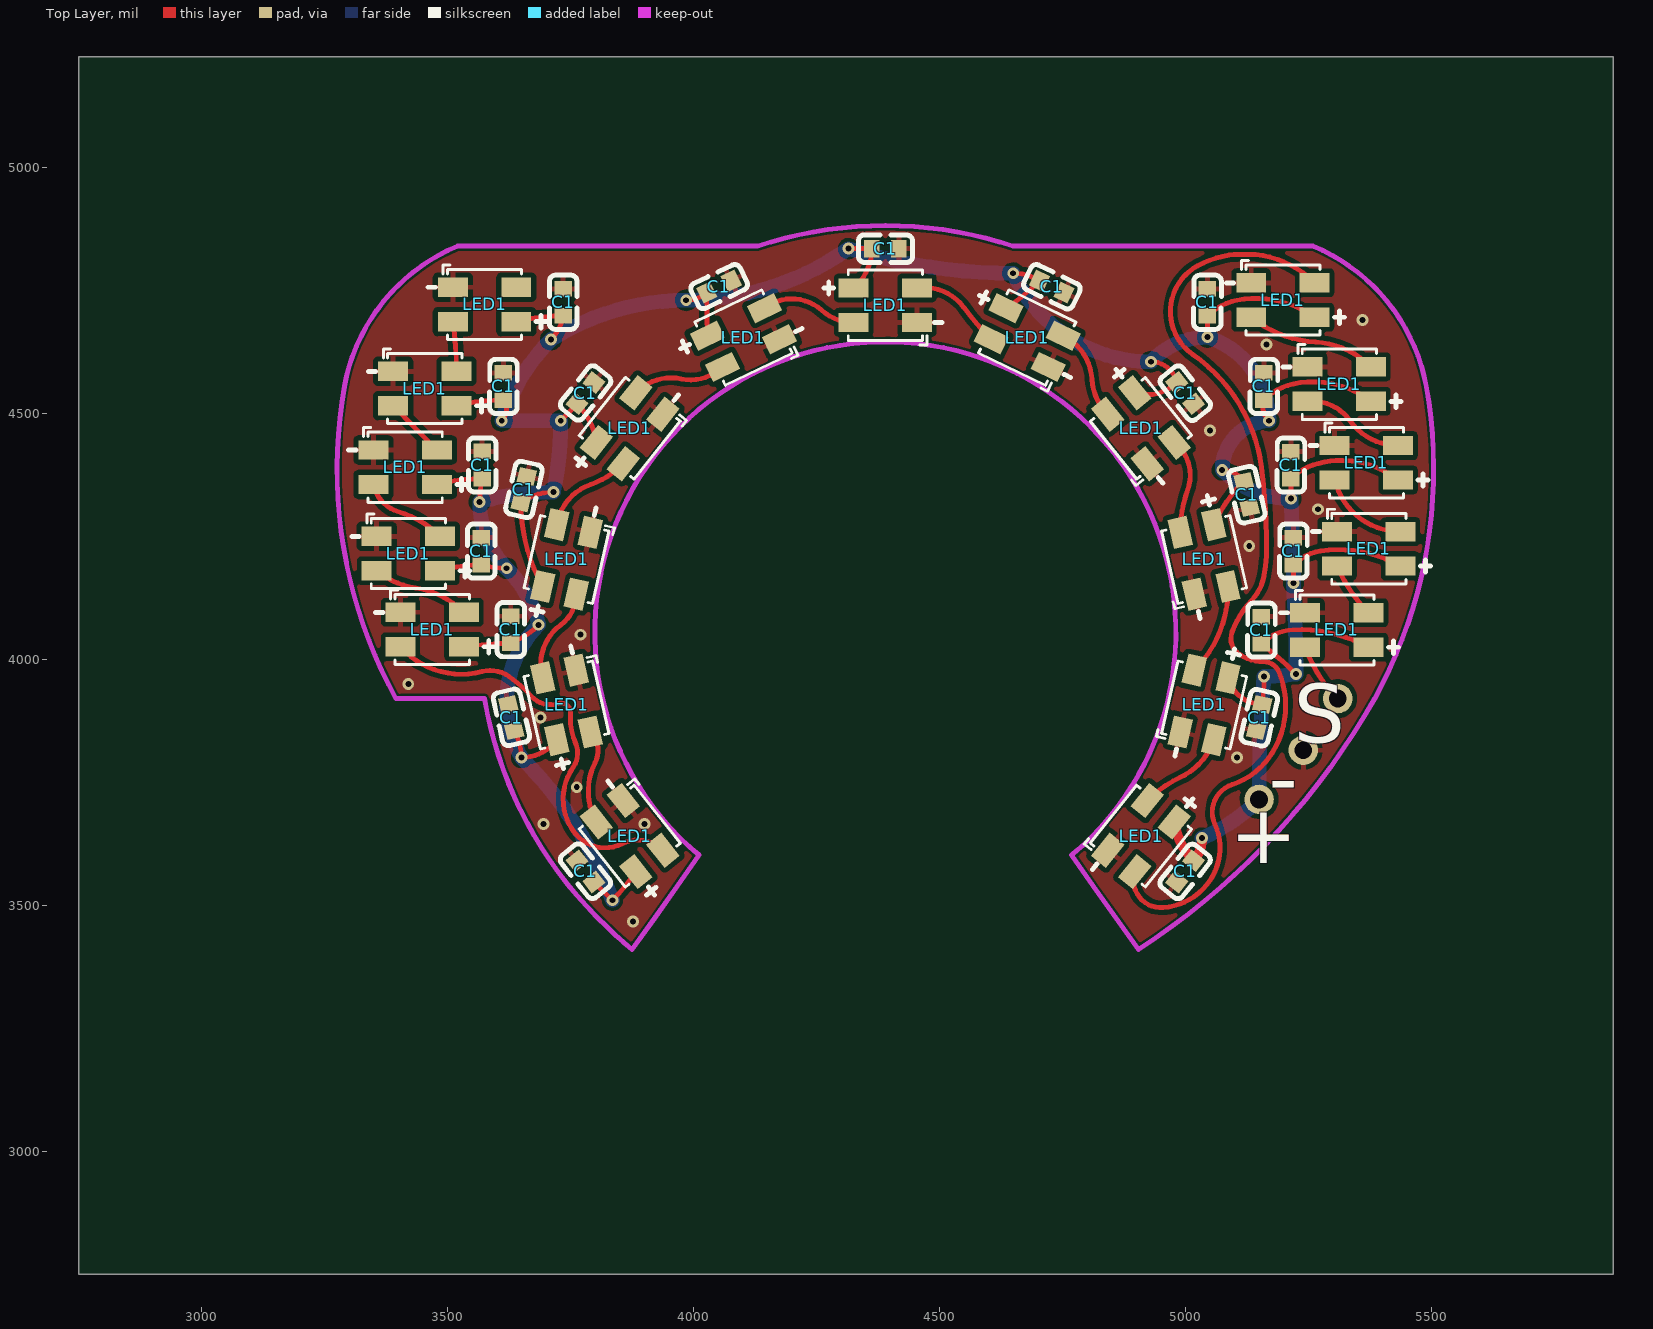
[diagram p0: Top Layer view]
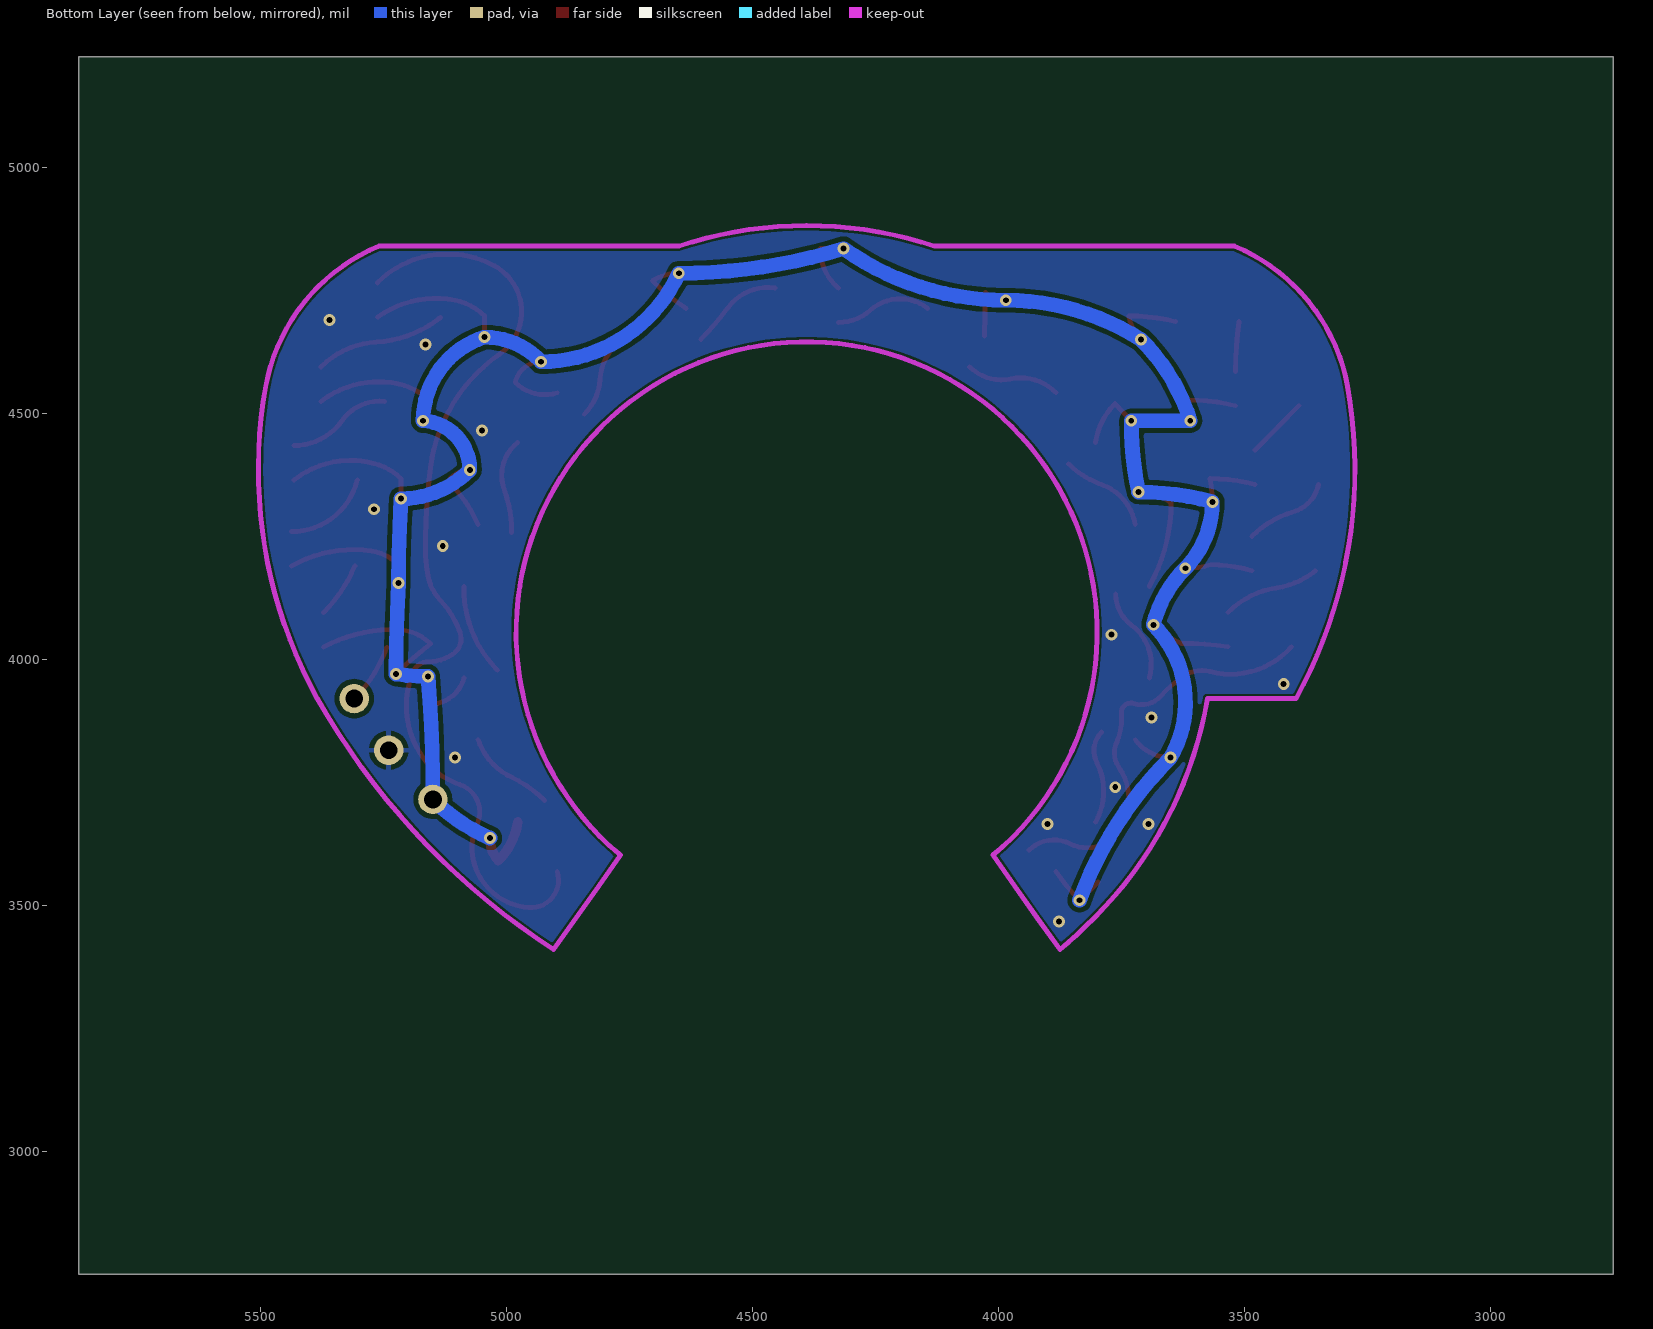
[diagram p1: Bottom Layer view, seen from below]
# Altium PCB MISC89036.pcbdoc
Units mil, origin at the board's own origin, x right, y up, seen from the top; angles counter-clockwise.
Board outline 3120 x 2475.23 mil, 2 copper layers (Top Layer, Bottom Layer), stack 62.206 mil thick; 42 components, 2 nets, 129 pads, 34 vias.

## Layer stack, top to bottom
Top Solder Mask Layer: solder mask 0.394, Dk 3.3
Top Layer: signal copper 1.379
Dielectric1: surface 59.449, FR4, Dk 4.5
Bottom Layer: signal copper 1.378
Bottom Solder Mask Layer: solder mask 0.394, Dk 3.3

## Board outline
5870,2750 2750,2750 2750,5225.23 5870,5225.23

## Design rules (kind name [scope] priority, off if disabled: settings)
BoardOutlineClearance copperThickness2oz_1 [All] p2 off: genericclearance=7.99 ignorepadtopadclearanceinfootprint=FALSE except(0: Arc-SplitContinuation Track-SplitContinuation SMDPad-SplitContinuation THPad-SplitContinuation Via-SplitContinuation Fill-SplitContinuation Region-SplitContinuation Poly-SplitContinuation Text-SplitContinuation Hole-SplitContinuation; 5.98: Arc-CutoutEdge Track-CutoutEdge SMDPad-CutoutEdge THPad-CutoutEdge Via-CutoutEdge Text-CutoutEdge; 6.9: Hole-OutlineEdge Hole-CutoutEdge; 10: Poly-OutlineEdge Poly-CutoutEdge; 11.81: Arc-OutlineEdge Track-OutlineEdge SMDPad-OutlineEdge THPad-OutlineEdge Via-OutlineEdge Fill-OutlineEdge Region-OutlineEdge Text-OutlineEdge Fill-CutoutEdge Region-CutoutEdge)
BoardOutlineClearance Plane_innerPlane_1 [All] p4 off: genericclearance=4.02 ignorepadtopadclearanceinfootprint=FALSE except(0: Arc-SplitContinuation Track-SplitContinuation SMDPad-SplitContinuation THPad-SplitContinuation Via-SplitContinuation Fill-SplitContinuation Region-SplitContinuation Poly-SplitContinuation Text-SplitContinuation Hole-SplitContinuation; 5.98: Arc-CutoutEdge Track-CutoutEdge SMDPad-CutoutEdge THPad-CutoutEdge Via-CutoutEdge Text-CutoutEdge; 6.9: Hole-OutlineEdge Hole-CutoutEdge; 10: Poly-OutlineEdge Poly-CutoutEdge; 11.81: Arc-OutlineEdge Track-OutlineEdge SMDPad-OutlineEdge THPad-OutlineEdge Via-OutlineEdge Fill-OutlineEdge Region-OutlineEdge Text-OutlineEdge Fill-CutoutEdge Region-CutoutEdge)
BoardOutlineClearance Copper_copperRegion_1 [All] p6 off: genericclearance=4.02 ignorepadtopadclearanceinfootprint=FALSE except(0: Arc-SplitContinuation Track-SplitContinuation SMDPad-SplitContinuation THPad-SplitContinuation Via-SplitContinuation Fill-SplitContinuation Region-SplitContinuation Poly-SplitContinuation Text-SplitContinuation Hole-SplitContinuation; 5.98: Arc-CutoutEdge Track-CutoutEdge SMDPad-CutoutEdge THPad-CutoutEdge Via-CutoutEdge Text-CutoutEdge; 6.9: Hole-OutlineEdge Hole-CutoutEdge; 10: Poly-OutlineEdge Poly-CutoutEdge; 11.81: Arc-OutlineEdge Track-OutlineEdge SMDPad-OutlineEdge THPad-OutlineEdge Via-OutlineEdge Fill-OutlineEdge Region-OutlineEdge Text-OutlineEdge Fill-CutoutEdge Region-CutoutEdge)
BoardOutlineClearance copperThickness1oz_1 [All] p8: genericclearance=4.02 ignorepadtopadclearanceinfootprint=FALSE except(0: Arc-SplitContinuation Track-SplitContinuation SMDPad-SplitContinuation THPad-SplitContinuation Via-SplitContinuation Fill-SplitContinuation Region-SplitContinuation Poly-SplitContinuation Text-SplitContinuation Hole-SplitContinuation; 5.98: Arc-CutoutEdge Track-CutoutEdge SMDPad-CutoutEdge THPad-CutoutEdge Via-CutoutEdge Text-CutoutEdge; 6.9: Hole-OutlineEdge Hole-CutoutEdge; 10: Poly-OutlineEdge Poly-CutoutEdge; 11.81: Arc-OutlineEdge Track-OutlineEdge SMDPad-OutlineEdge THPad-OutlineEdge Via-OutlineEdge Fill-OutlineEdge Region-OutlineEdge Text-OutlineEdge Fill-CutoutEdge Region-CutoutEdge)
Clearance copperThickness2oz [All] p1 off: gap=7.99 ignorepadtopadclearanceinfootprint=FALSE except(5.98: SMDPad-Track SMDPad-SMDPad THPad-Track SMDPad-THPad THPad-THPad Track-Via SMDPad-Via THPad-Via Via-Via Fill-SMDPad Region-SMDPad Fill-THPad Region-THPad Fill-Via Region-Via Fill-Fill Fill-Region Region-Region Arc-Track Arc-SMDPad Arc-THPad Arc-Via Fill-Arc Region-Arc Arc-Arc Text-Track SMDPad-Text Text-THPad Text-Via Fill-Text Region-Text Arc-Text Text-Text; 6.9: Hole-Track Hole-SMDPad Hole-THPad Hole-Via Fill-Hole Region-Hole Hole-Arc Hole-Text; 10: Poly-Track Poly-SMDPad Poly-THPad Poly-Via Poly-Fill Poly-Region Poly-Poly Poly-Arc Poly-Text Poly-Hole; 11.81: Fill-Track Region-Track)
Clearance Plane_innerPlane [All] p3 off: gap=4.02 ignorepadtopadclearanceinfootprint=FALSE except(5.98: SMDPad-Track SMDPad-SMDPad THPad-Track SMDPad-THPad THPad-THPad Track-Via SMDPad-Via THPad-Via Via-Via Fill-SMDPad Region-SMDPad Fill-THPad Region-THPad Fill-Via Region-Via Fill-Fill Fill-Region Region-Region Arc-Track Arc-SMDPad Arc-THPad Arc-Via Fill-Arc Region-Arc Arc-Arc Text-Track SMDPad-Text Text-THPad Text-Via Fill-Text Region-Text Arc-Text Text-Text; 6.9: Hole-Track Hole-SMDPad Hole-THPad Hole-Via Fill-Hole Region-Hole Hole-Arc Hole-Text; 10: Poly-Track Poly-SMDPad Poly-THPad Poly-Via Poly-Fill Poly-Region Poly-Poly Poly-Arc Poly-Text Poly-Hole; 11.81: Fill-Track Region-Track)
Clearance Copper_copperRegion [All] p5 off: gap=4.02 ignorepadtopadclearanceinfootprint=FALSE except(5.98: SMDPad-Track SMDPad-SMDPad THPad-Track SMDPad-THPad THPad-THPad Track-Via SMDPad-Via THPad-Via Via-Via Fill-SMDPad Region-SMDPad Fill-THPad Region-THPad Fill-Via Region-Via Fill-Fill Fill-Region Region-Region Arc-Track Arc-SMDPad Arc-THPad Arc-Via Fill-Arc Region-Arc Arc-Arc Text-Track SMDPad-Text Text-THPad Text-Via Fill-Text Region-Text Arc-Text Text-Text; 6.9: Hole-Track Hole-SMDPad Hole-THPad Hole-Via Fill-Hole Region-Hole Hole-Arc Hole-Text; 10: Poly-Track Poly-SMDPad Poly-THPad Poly-Via Poly-Fill Poly-Region Poly-Poly Poly-Arc Poly-Text Poly-Hole; 11.81: Fill-Track Region-Track)
Clearance copperThickness1oz [All] p7: gap=4.02 ignorepadtopadclearanceinfootprint=FALSE except(5.98: SMDPad-Track SMDPad-SMDPad THPad-Track SMDPad-THPad THPad-THPad Track-Via SMDPad-Via THPad-Via Via-Via Fill-SMDPad Region-SMDPad Fill-THPad Region-THPad Fill-Via Region-Via Fill-Fill Fill-Region Region-Region Arc-Track Arc-SMDPad Arc-THPad Arc-Via Fill-Arc Region-Arc Arc-Arc Text-Track SMDPad-Text Text-THPad Text-Via Fill-Text Region-Text Arc-Text Text-Text; 6.9: Hole-Track Hole-SMDPad Hole-THPad Hole-Via Fill-Hole Region-Hole Hole-Arc Hole-Text; 10: Poly-Track Poly-SMDPad Poly-THPad Poly-Via Poly-Fill Poly-Region Poly-Poly Poly-Arc Poly-Text Poly-Hole; 11.81: Fill-Track Region-Track)
DiffPairsRouting differentialPair [All] p1: maxlimit=6 minlimit=6 mostfreqgap=6 toplayer_minwidth=5 toplayer_prefwidth=10 toplayer_maxwidth=100 toplayer_mingap=6 toplayer_prefgap=6 toplayer_maxgap=6 bottomlayer_minwidth=5 bottomlayer_prefwidth=10 bottomlayer_maxwidth=100 bottomlayer_mingap=6 bottomlayer_prefgap=6 bottomlayer_maxgap=6 maxuncoupledlength=10
HoleToHoleClearance otherClearance [All] p1: gap=11.81 allowstackedmicrovias=TRUE
Length netLength [All] p1: minlimit=0 maxlimit=0
PasteMaskExpansion pasteMaskExpansion [All] p1: expansion=0
PlaneConnect innerPlane [All] p1: planeconnectstyle=Relief reliefexpansion=20 reliefentries=4 reliefconductorwidth=10 reliefairgap=10
PolygonConnect copperRegion [All] p1: connectstyle=Relief reliefconductorwidth=10 reliefentries=4 polygonreliefangle="90 Angle" airgapwidth=10 via.connectstyle=Relief via.reliefconductorwidth=10 via.reliefentries=4 via.polygonreliefangle="90 Angle" via.airgapwidth=10
RoutingVias viaSize [All] p1: holewidth=12.01 width=24.02 viastyle="Through Hole" minholewidth=11.81 minwidth=19.68 maxholewidth=248.03 maxwidth=393.7
SolderMaskExpansion solderMaskExpansion [IsVia] p1: expansion=-1000 istentingtop=TRUE
SolderMaskExpansion solderMaskExpansion [All] p2: expansion=2 istentingtop=FALSE
Width copperThickness2oz_2 [All] p1 off: maxlimit=100 minlimit=8 preferedwidth=10
Width copperThickness1oz_2 [All] p2: maxlimit=100 minlimit=5 preferedwidth=10

## Components (designator, comment, footprint, x,y, rotation, side; value= is the part's Value field where it differs from the comment)
C1 "100nF" C0603#1 4390,4835.23 r180 top
C1 "100nF" C0603#2 4051.57,4757.99 r205.7 top
C1 "100nF" C0603#3 3780.17,4541.55 r231.4 top
C1 "100nF" C0603#4 3655,4345.23 r257.1 top
C1 "100nF" C0603#5 3629.56,3881.66 r282.9 top
C1 "100nF" C0603#6 3780.17,3568.91 r308.6 top
C1 "100nF" C0603#3 4999.83,3568.91 r51.4 top
C1 "100nF" C0603#4 5150.44,3881.66 r77.1 top
C1 "100nF" C0603#5 5125,4335.23 r102.9 top
C1 "100nF" C0603#6 4999.83,4541.55 r128.6 top
C1 "100nF" C0603#7 4728.43,4757.99 r154.3 top
C1 "100nF" C0603#1 3734.79,4725.92 r270 top
C1 "100nF" C0603#1 3613.31,4554.92 r270 top
C1 "100nF" C0603#1 3570,4395.23 r270 top
C1 "100nF" C0603#1 3568.31,4219.92 r270 top
C1 "100nF" C0603#1 3628.31,4060.12 r270 top
C1 "100nF" C0603#1 5045,4725.92 r270 top
C1 "100nF" C0603#1 5159.72,4554.92 r270 top
C1 "100nF" C0603#1 5214.72,4394.92 r270 top
C1 "100nF" C0603#1 5219.72,4219.92 r270 top
C1 "100nF" C0603#1 5154.72,4059.23 r270 top
LED1 "WS2812B-Mini" LED-SMD_4P-L3.5-W3.5-TL_WS2812B#1 4390,4720.23 r0 top
LED1 "WS2812B-Mini" LED-SMD_4P-L3.5-W3.5-TL_WS2812B#2 4101.47,4654.37 r25.7 top
LED1 "WS2812B-Mini" LED-SMD_4P-L3.5-W3.5-TL_WS2812B#3 3870.08,4469.85 r51.4 top
LED1 "WS2812B-Mini" LED-SMD_4P-L3.5-W3.5-TL_WS2812B#4 3741.67,4203.21 r77.1 top
LED1 "WS2812B-Mini" LED-SMD_4P-L3.5-W3.5-TL_WS2812B#5 3741.67,3907.25 r102.9 top
LED1 "WS2812B-Mini" LED-SMD_4P-L3.5-W3.5-TL_WS2812B#6 3870.08,3640.61 r128.6 top
LED1 "WS2812B-Mini" LED-SMD_4P-L3.5-W3.5-TL_WS2812B#3 4909.92,3640.61 r231.4 top
LED1 "WS2812B-Mini" LED-SMD_4P-L3.5-W3.5-TL_WS2812B#4 5038.33,3907.25 r257.1 top
LED1 "WS2812B-Mini" LED-SMD_4P-L3.5-W3.5-TL_WS2812B#5 5038.33,4203.21 r282.9 top
LED1 "WS2812B-Mini" LED-SMD_4P-L3.5-W3.5-TL_WS2812B#6 4909.92,4469.85 r308.6 top
LED1 "WS2812B-Mini" LED-SMD_4P-L3.5-W3.5-TL_WS2812B#7 4678.53,4654.37 r334.3 top
LED1 "WS2812B-Mini" LED-SMD_4P-L3.5-W3.5-TL_WS2812B#1 3575,4721.73 r180 top
LED1 "WS2812B-Mini" LED-SMD_4P-L3.5-W3.5-TL_WS2812B#1 3453.52,4550.73 r180 top
LED1 "WS2812B-Mini" LED-SMD_4P-L3.5-W3.5-TL_WS2812B#1 3413.52,4390.73 r180 top
LED1 "WS2812B-Mini" LED-SMD_4P-L3.5-W3.5-TL_WS2812B#1 3420,4215.23 r180 top
LED1 "WS2812B-Mini" LED-SMD_4P-L3.5-W3.5-TL_WS2812B#1 3468.52,4060.73 r180 top
LED1 "WS2812B-Mini" LED-SMD_4P-L3.5-W3.5-TL_WS2812B#1 5198.52,4730.73 r180 top
LED1 "WS2812B-Mini" LED-SMD_4P-L3.5-W3.5-TL_WS2812B#1 5313.24,4559.73 r180 top
LED1 "WS2812B-Mini" LED-SMD_4P-L3.5-W3.5-TL_WS2812B#1 5368.24,4399.73 r180 top
LED1 "WS2812B-Mini" LED-SMD_4P-L3.5-W3.5-TL_WS2812B#1 5373.24,4224.73 r180 top
LED1 "WS2812B-Mini" LED-SMD_4P-L3.5-W3.5-TL_WS2812B#1 5308.24,4059.73 r180 top

## Footprints (in the part's own frame and the unit in brackets; to place one, negate y for a bottom-side part, rotate by r counter-clockwise, add the part's x,y. Pads: shape width x height; smd on the part's side, far side on the other; paste and mask are expansions set on the pad)
C0603#1 [mm]
  rect 0.8x0.9 smd: 1(-0.7,0) 2(0.7,0)
  silkscreen extent -1.41,-0.71 1.39,0.72
C0603#2 [mm]
  rect 0.8x0.9 smd rot 0.01: 1(-0.7,0) 2(0.7,0)
  silkscreen extent -1.41,-0.71 1.39,0.72
C0603#3 [mm]
  rect 0.8x0.9 smd rot 0.03: 1(-0.7,0) 2(0.7,0)
  silkscreen extent -1.41,-0.71 1.39,0.72
C0603#4 [mm]
  rect 0.8x0.9 smd rot 0.04: 1(-0.7,-0.001) 2(0.7,0.001)
  silkscreen extent -1.41,-0.71 1.39,0.72
C0603#5 [mm]
  rect 0.8x0.9 smd rot 179.96: 1(-0.7,0.001) 2(0.7,-0.001)
  silkscreen extent -1.41,-0.71 1.39,0.72
C0603#6 [mm]
  rect 0.8x0.9 smd rot 179.97: 1(-0.7,0) 2(0.7,0)
  silkscreen extent -1.41,-0.71 1.39,0.72
C0603#7 [mm]
  rect 0.8x0.9 smd rot 179.99: 1(-0.7,0) 2(0.7,0)
  silkscreen extent -1.41,-0.71 1.39,0.72
LED-SMD_4P-L3.5-W3.5-TL_WS2812B#1 [mm]
  rect 1.545x0.997 smd: 1(-1.638,0.89) 2(-1.638,-0.89) 3(1.638,-0.89) 4(1.638,0.89)
  silkscreen extent -3.17,-2.04 2.92,1.82
LED-SMD_4P-L3.5-W3.5-TL_WS2812B#2 [mm]
  rect 1.545x0.997 smd rot 0.01: 1(-1.638,0.89) 2(-1.637,-0.89) 3(1.638,-0.89) 4(1.637,0.89)
  silkscreen extent -3.18,-2.04 2.92,1.82
LED-SMD_4P-L3.5-W3.5-TL_WS2812B#3 [mm]
  rect 1.545x0.997 smd rot 0.03: 1(-1.638,0.889) 2(-1.637,-0.891) 3(1.638,-0.889) 4(1.637,0.891)
  silkscreen extent -3.18,-2.04 2.92,1.82
LED-SMD_4P-L3.5-W3.5-TL_WS2812B#4 [mm]
  rect 1.545x0.997 smd rot 0.04: 1(-1.638,0.889) 2(-1.637,-0.891) 3(1.638,-0.889) 4(1.637,0.891)
  silkscreen extent -3.18,-2.04 2.92,1.82
LED-SMD_4P-L3.5-W3.5-TL_WS2812B#5 [mm]
  rect 1.545x0.997 smd rot 179.96: 1(-1.637,0.891) 2(-1.638,-0.889) 3(1.637,-0.891) 4(1.638,0.889)
  silkscreen extent -3.17,-2.05 2.92,1.82
LED-SMD_4P-L3.5-W3.5-TL_WS2812B#6 [mm]
  rect 1.545x0.997 smd rot 179.97: 1(-1.637,0.891) 2(-1.638,-0.889) 3(1.637,-0.891) 4(1.638,0.889)
  silkscreen extent -3.17,-2.05 2.92,1.82
LED-SMD_4P-L3.5-W3.5-TL_WS2812B#7 [mm]
  rect 1.545x0.997 smd rot 179.99: 1(-1.637,0.89) 2(-1.638,-0.89) 3(1.637,-0.89) 4(1.638,0.89)
  silkscreen extent -3.17,-2.05 2.92,1.82

## Free pads (board coordinates)
  round 60 hole 36: 1(5310,3920.23) 2(5240,3815.23) 3(5150,3715.23)

## Via types
v1: diameter 24.02, hole 12, Top Layer to Bottom Layer, 34 vias

## Nets (pads, with @x,y where several pads share a name; then routed paths per layer and width w, separated by ;. In a path a pad name is that pad's centre, name@x,y a point inside that pad or via, vN(x,y) a via of type N, cw(c..) or ccw(c..) an arc to the next point about the centre after c; other vN are vias at no path point)
GND: C1.1 LED1.3 pad.2
  other v1: 3876.72,3466.78 3695,3665.23 3900,3665.23 3762.5,3740.08 5105,3800.23 3688.61,3881.98 3420,3950.23 3770,4050.23 5130,4230.23 5270,4305.23 5050,4465.23 5165,4640.23 5360,4690.23
VCC: C1.2 LED1.1 pad.3 | length 8199.7
  Top Layer w10: LED1.1@3477.99,4355.69 cw(c3570,4008.37) 3570,4367.67 ccw(c3792.56,4320.23) v1(3565,4320.23) ; LED1.1@3484.47,4180.19 cw(c3568.31,3897.61) 3568.31,4192.36 ccw(c3620,4376.03) v1(3620,4185.23) ; LED1.1@3517.99,4515.69 cw(c3613.31,4132.43) 3613.31,4527.36 cw(c3587,4508.23) v1(3610,4485.23) ; LED1.1@3532.99,4025.69 cw(c3628.31,3367.9) 3628.31,4032.56 ccw(c3563.21,4192.02) v1(3685,4070.23) ; C1.2@3635.69,3854.79 cw(c3538.82,3800.23) v1(3650,3800.23) ccw(c3650,3889.4) LED1.1@3721.86,3836.6 ; LED1.1@3639.47,4686.69 cw(c3734.79,4303.43) 3734.79,4698.36 cw(c3647.22,4713.01) v1(3710,4650.23) ; LED1.1@3693.17,4148.15 cw(c3998.02,4318.36) 3648.87,4318.36 cw(c3715,4229.3) v1(3715,4340.23) ; v1(3730,4485.23) ccw(c3087.07,5128.16) 3762.99,4520 cw(c3664.08,4421.1) LED1.1@3802.49,4441.29 ; C1.2@3797.35,3547.36 v1(3835,3510.23) ccw(c3558.2,3787.03) LED1.1@3882.88,3568.36 ; v1(3985,4730.23) ccw(c3985,4793.27) 4026.74,4746.03 ccw(c6722.47,4746.03) LED1.1@4028.18,4657.97 ; v1(4315,4835.23) 4362.44,4835.23 cw(c4257.37,4835.23) LED1.1@4325.53,4755.27 ; LED1.1@4635.65,4713.92 ccw(c4378.31,5095.24) 4703.6,4769.94 ccw(c4650,4683.62) v1(4650,4785.23) ; LED1.1@4897.12,4542.1 ccw(c4922.55,4623.19) 4982.65,4563.1 ccw(c4930,4551.27) v1(4930,4605.23) ; v1(5045,4655.23) 5045,4698.36 cw(c5127.02,4616.34) 5105,4730.23 cw(c5143.85,4529.32) LED1.1@5262.99,4695.69 ; LED1.1@5058.14,4273.86 cw(c5327.35,4153.61) 5118.87,4362.1 ccw(c5075,4332.07) v1(5075,4385.23) ; LED1.1@5086.83,3962.31 ccw(c5156.58,3980.64) 5156.58,3908.53 ccw(c4688.82,3965.23) v1(5160,3965.23) ; v1(5170,4485.23) cw(c5199.53,4514.76) 5159.72,4527.36 cw(c5245.68,4441.4) 5220,4560.23 cw(c5260.56,4372.54) 5248.12,4564.16 5263.01,4564.16 cw(c5263.01,4344.26) 5282.97,4563.25 cw(c5260.56,4372.54) LED1.1@5377.71,4524.69 ; v1(5214.71,4326.74) 5214.72,4367.36 cw(c5295.86,4286.22) 5260,4395.23 cw(c5317.92,4219.17) 5306.48,4404.16 5319.36,4404.16 cw(c5319.36,4178.94) 5339.32,4403.27 cw(c5317.92,4219.17) LED1.1@5432.71,4364.69 ; v1(5220,4155.23) 5219.72,4192.36 cw(c5289.61,4122.47) 5275,4220.23 cw(c5312.33,3970.41) LED1.1@5437.71,4189.69 ; v1(5225,3970.23) ccw(c4732.33,3477.56) 5154.72,4031.67 cw(c5223.85,3962.54) 5220,4060.23 cw(c5231.65,3764.45) LED1.1@5372.71,4024.69
  Top Layer w20: LED1.1@4977.51,3669.17 ccw(c5115.92,3689.36) 5017.01,3590.45 ccw(c4963.07,3636.69) v1(5034.11,3636.69)
  Bottom Layer w30: v1(3835,3510.23) ccw(c3086.55,3236.78) v1(3650,3800.23) cw(c3842.71,3912.52) v1(3685,4070.23) ccw(c3445.5,4010.73) v1(3620,4185.23) cw(c3758.18,4320.23) v1(3565,4320.23) cw(c3715,3767.73) v1(3715,4340.23) ccw(c3021.67,4485.23) v1(3730,4485.23) v1(3610,4485.23) cw(c3996.35,4363.88) v1(3710,4650.23) cw(c3985,4217.57) v1(3985,4730.23) ccw(c3985,5301.3) v1(4315,4835.23) ccw(c4650,5932.48) v1(4650,4785.23) ccw(c4930,4913.01) v1(4930,4605.23) cw(c5045,4497.98) v1(5045,4655.23) cw(c4991.9,4485.23) v1(5170,4485.23) ccw(c5175.13,4385.23) v1(5075,4385.23) ccw(c5214.71,4522.82) v1(5214.71,4326.74) cw(c2439.31,4155.23) v1(5220,4155.23) cw(c1799.98,3970.23) v1(5225,3970.23) cw(c5160,4390.23) v1(5160,3965.23) ccw(c8280.01,3715.23) pad.3 cw(c4887.59,3977.64) v1(5034.11,3636.69)
pads on no net: LED1.2 LED1.4
copper on no net: | length 6255.3
  Top Layer w10: 3349.05,4355.69 ccw(c3420.27,4369.98) 3400,4300.23 cw(c3344.93,4110.73) 3484.47,4250.27 ; 3355.53,4180.19 ccw(c3459.68,4309.14) 3435,4145.23 cw(c3408.86,3971.64) 3532.99,4095.77 ; 3389.05,4515.69 3477.99,4425.77 ; 3404.05,4025.69 ccw(c3527.99,4135.16) 3570,3975.23 cw(c3586.79,3911.32) 3625,3965.23 cw(c3466.49,3741.6) 3670,3925.23 ccw(c3709.19,3960.59) 3725,3910.23 cw(c3730.78,3891.83) 3750,3890.23 ccw(c3873.47,3879.97) 3760,3830.23 cw(c3713.1,3809.67) 3755,3780.23 ccw(c3846.38,3716.02) 3760,3645.23 ccw(c3819.95,3694.36) 3855,3625.23 cw(c3887.25,3561.63) 3937.67,3612.05 ; 3510.53,4686.69 cw(c2831.9,4585.77) 3517.99,4585.77 ; 3693.17,3962.31 cw(c3789.33,3989.73) 3730,4070.23 ccw(c3684.06,4132.56) 3761.49,4132.56 ; 3721.86,4273.86 cw(c3824.57,4257.06) 3790,4355.23 ccw(c3730.4,4524.48) 3857.28,4397.6 ; 3790.18,3852.2 cw(c3752.44,3814.45) 3800,3790.23 ccw(c3914.28,3732.02) 3802.49,3669.17 ; 3882.88,4542.1 cw(c3954.13,4473.68) 3975,4570.23 ccw(c3994.23,4659.19) 4058.59,4594.83 ; 4144.35,4713.92 cw(c4199.98,4643.16) 4260,4710.23 ccw(c4325.53,4783.46) 4325.53,4685.19 ; 4454.47,4755.27 cw(c4468.99,4655.94) 4550,4715.23 ccw(c4996.52,5042.05) 4605.24,4650.78 ; 4751.82,4657.97 cw(c4705.18,4563.88) 4810,4570.23 ccw(c4920.86,4576.94) 4842.33,4498.41 ; 4897.12,3568.36 ccw(c4950.7,3551.3) 4955,3495.23 ccw(c4945.33,3621.49) 5050,3550.23 ccw(c4952.43,3616.65) 5060,3665.23 cw(c5113.6,3689.44) 5095,3745.23 ccw(c5046.94,3889.4) 5170,3800.23 ccw(c5024.77,3905.47) 5190,3975.23 ccw(c5159.85,3962.5) 5160,3995.23 cw(c5160.43,4087.51) 5110,4010.23 cw(c5130.85,4042.18) 5095,4055.23 cw(c5273.23,3990.36) 5135,4120.23 ccw(c5063.9,4187.03) 5160,4170.23 ccw(c4752.21,4241.52) 5165,4210.23 ccw(c3979.45,4234.64) 5155,4390.23 ccw(c4824.13,4346.44) 5015,4620.23 cw(c5075.59,4707.14) 5025,4800.23 cw(c5120.93,4623.71) 5089.15,4822.08 cw(c5109.06,4674.38) 5109.06,4823.42 5142.81,4823.42 cw(c5120.93,4623.71) 5262.99,4765.77 ; 4922.72,3712.86 cw(c5092.73,3542.85) 4990,3760.23 ccw(c4933.95,3878.82) 5058.14,3836.6 ; 4977.51,4441.29 cw(c4924.59,4374.18) 5005,4345.23 ccw(c5246.53,4258.26) 4989.82,4258.26 ; 5018.51,3977.9 ccw(c4853.43,4142.99) 5086.83,4148.15 ; 5134.05,4695.69 ccw(c5277.93,4873.93) 5265,4645.23 cw(c5255.22,4472.28) 5377.71,4594.77 ; 5243.77,4024.69 ccw(c5510.09,4120.32) 5310,3920.23 ; 5248.77,4524.69 cw(c5257.76,4430.39) 5335,4485.23 ccw(c5432.71,4554.6) 5432.71,4434.77 ; 5303.77,4364.69 ccw(c5437.71,4397.72) 5437.71,4259.77 ; 5308.77,4189.69 ccw(c5584.11,4306.17) 5372.71,4094.77

## Polygon pours and split planes (outlines as drawn)
GND on Bottom Layer (solid, remove dead copper, pour order 2): 3255,4895.23 3255,3365.23 5545,3365.23 5545,4895.23
GND on Top Layer (solid, remove dead copper, pour order 0): 3230,4925.23 3230,3355.23 5620,3355.23 5620,4925.23

## Keep-outs
Board Outline Layer:
  lines w10: 3290,4555.23 cw(c3667.23,4486.1) 3520,4840.23 4130,4840.23 cw(c4388.75,4059.71) 4390,4882 cw(c4391.25,4059.71) 4650,4840.23 5260,4840.23 cw(c5112.77,4486.1) 5490,4555.23 cw(c4539.27,4386.26) 5385,3920.23 cw(c4095.58,4652.92) 4905,3410.23 cw(c11995.54,8597.12) 4768.6,3602.03 ccw(c4437.73,4012.75) 4790,3620.23 ccw(c4390,4055) 3990,3620.23 ccw(c4342.27,4012.75) 4011.4,3602.03 cw(c-3215.54,8597.12) 3875,3410.23 cw(c4228.05,3852.78) 3825,3455.23 cw(c4387.42,4057.31) 3575,3920.23 3395,3920.23 cw(c4240.73,4386.26) 3290,4555.23

## Silkscreen, mask and mechanical layers (free items; w line width, h text height)
Top Silkscreen Layer:
  text "S" at 5220,3830.23 h120
  text "-" at 5170,3700.23 h120
  text "+" at 5090,3585.23 h120
Document Layer:
  circle w10: c4390,4055.23 r590.55

## Dimensions
3280,4975.23 to 5505,4975.23 on Document Layer
3105,4910.23 to 3105,3350.23 on Document Layer